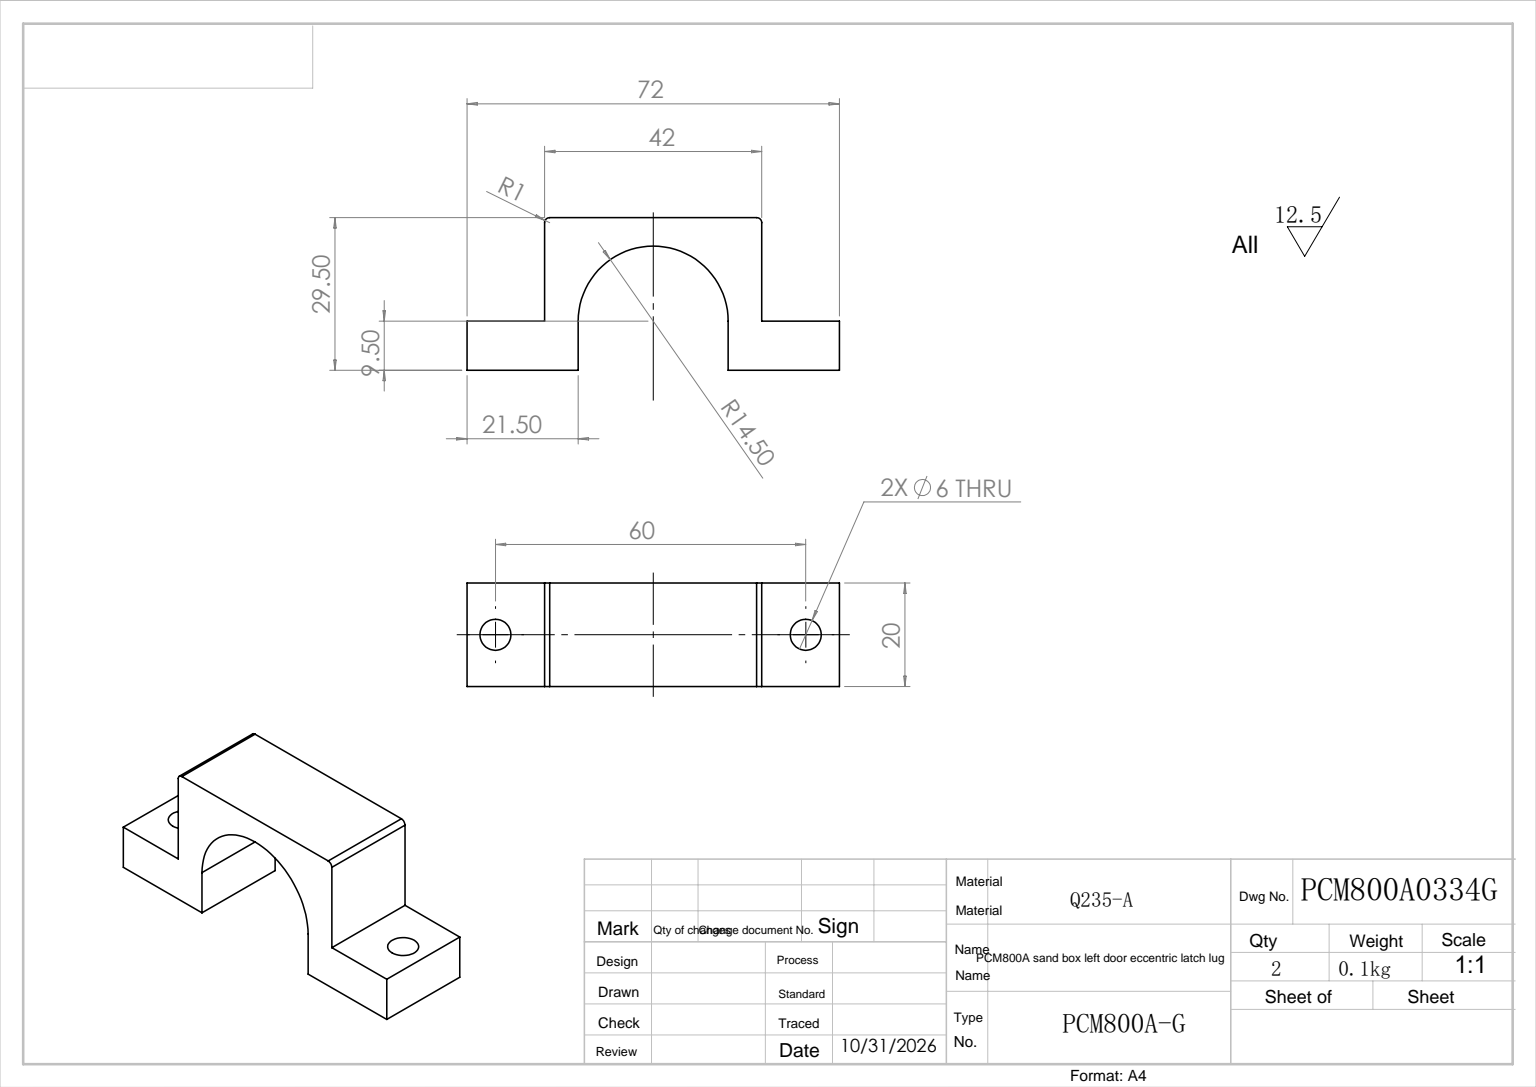
from build123d import *

# Parameters (mm, degrees)
EXTRUDE_1_DEPTH     = 20
FILLET_1_R          = 1
SKETCH_2_R          = 3
CUT_EXTRUDE_1_DEPTH = 78.356318423


with BuildPart() as part:
    # 草图1 → 凸台-拉伸1 (new body)
    with BuildSketch(Plane.XY):
        with BuildLine():
            Line((0, 0), (15, 0))
            Line((15, 0), (15, 20))
            Line((15, 20), (57, 20))
            Line((57, 20), (57, 0))
            Line((57, 0), (72, 0))
            Line((72, 0), (72, -9.5))
            Line((72, -9.5), (50.5, -9.5))
            Line((50.5, -9.5), (50.5, 0))
            ThreePointArc((50.5, 0), (36, 14.5), (21.5, 0))
            Line((21.5, 0), (21.5, -9.5))
            Line((21.5, -9.5), (0, -9.5))
            Line((0, -9.5), (0, 0))
        make_face()
    extrude(amount=EXTRUDE_1_DEPTH)

    # 圆角1
    fillet_1_edges = [part.edges().sort_by_distance(p)[0] for p in [
        (15, 20, 10),
        (57, 20, 10),
    ]]
    fillet(fillet_1_edges, radius=FILLET_1_R)

    # 草图2 → 切除-拉伸1 (cut, through all)
    with BuildSketch(Plane(origin=(0, 0, 0), x_dir=(1, 0, 0), z_dir=(0, 1, 0))):
        with Locations(Location((6.5, -10, 0), (0, 0, 270))):
            Circle(SKETCH_2_R)
        with Locations(Location((66.5, -10, 0), (0, 0, 270))):
            Circle(SKETCH_2_R)
    extrude(amount=-CUT_EXTRUDE_1_DEPTH, mode=Mode.SUBTRACT)


solid = part.part
